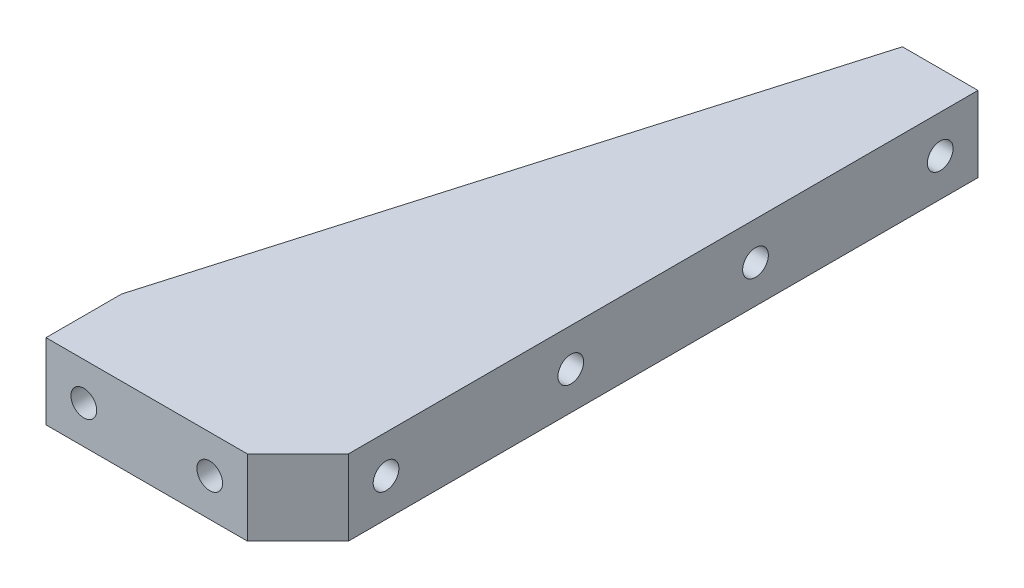
from build123d import *

# Parameters (mm, degrees)
EXTRUDE_1_DEPTH         = 30
HOLE_WIZARD_M12_1_D     = 10.2
HOLE_WIZARD_M12_1_DEPTH = 29.25
HOLE_WIZARD_M12_1_TIP   = 3.064389157
HOLE_WIZARD_M12_2_D     = 10.2
HOLE_WIZARD_M12_2_DEPTH = 29.25
HOLE_WIZARD_M12_2_TIP   = 3.064389157


with BuildPart() as part:
    # 草图1 → 凸台-拉伸1 (new body)
    with BuildSketch(Plane(origin=(0, 0, 0), x_dir=(1, 0, 0), z_dir=(0, 1, 0))):
        Polygon((0, 0), (0, -250), (-20, -270), (-100, -270), (-100, -240), (-30, 0), align=None)
    extrude(amount=EXTRUDE_1_DEPTH)

    # M12 螺纹孔1
    with Locations(Plane(origin=(0, 0, 0), x_dir=(0, 0, -1), z_dir=(1, 0, 0))):
        with Locations((-235, 15), (-15, 15), (-88.333333333, 15), (-161.666666667, 15)):
            Hole(HOLE_WIZARD_M12_1_D / 2, depth=HOLE_WIZARD_M12_1_DEPTH)
            with Locations((0, 0, -(HOLE_WIZARD_M12_1_DEPTH + HOLE_WIZARD_M12_1_TIP / 2))):  # 118° drill point
                Cone(0, HOLE_WIZARD_M12_1_D / 2, HOLE_WIZARD_M12_1_TIP, mode=Mode.SUBTRACT)

    # M12 螺纹孔2
    with Locations(Plane.XY.offset(270)):
        with Locations((-35, 15), (-85, 15)):
            Hole(HOLE_WIZARD_M12_2_D / 2, depth=HOLE_WIZARD_M12_2_DEPTH)
            with Locations((0, 0, -(HOLE_WIZARD_M12_2_DEPTH + HOLE_WIZARD_M12_2_TIP / 2))):  # 118° drill point
                Cone(0, HOLE_WIZARD_M12_2_D / 2, HOLE_WIZARD_M12_2_TIP, mode=Mode.SUBTRACT)


solid = part.part
